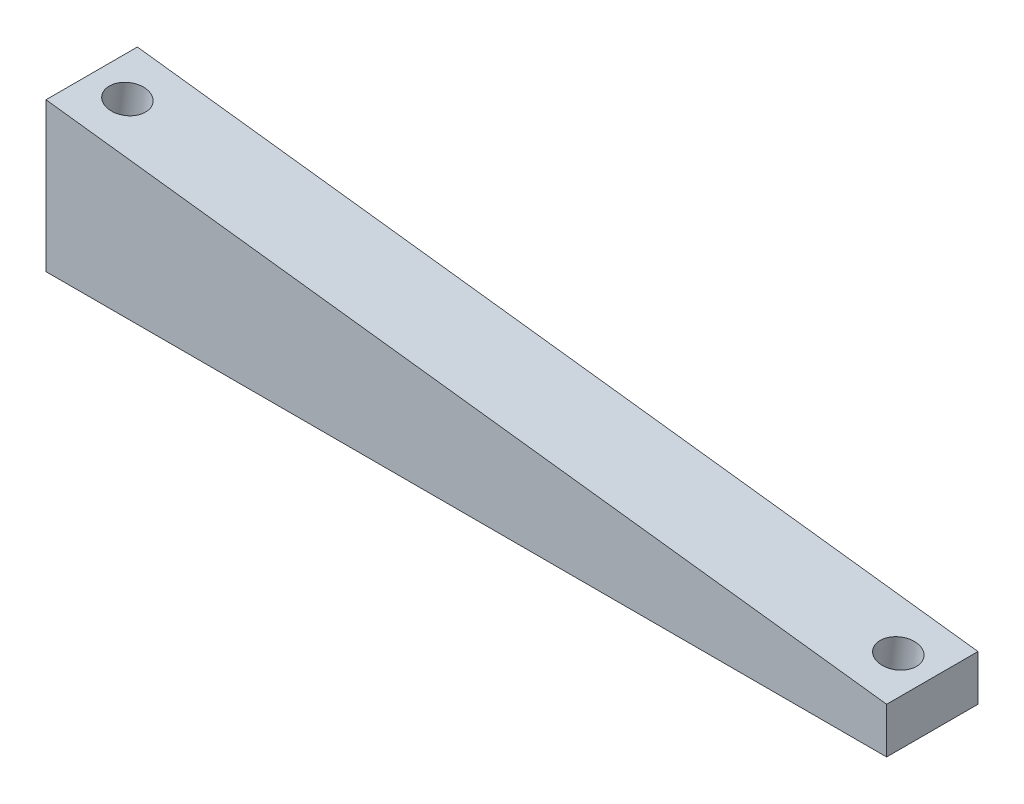
SolidWorks part; units mm, degrees
material "Plain Carbon Steel"
ref_plane "Front Plane" through (0, 0, 0) normal (0, 0, 1) x (1, 0, 0)
ref_plane "Top Plane" through (0, 0, 0) normal (0, 1, 0) x (1, 0, 0)
ref_plane "Right Plane" through (0, 0, 0) normal (1, 0, 0) x (0, 0, -1)
sketch "Sketch1" plane through (0, 0, 0) normal (0, 0, 1) x (1, 0, 0)
  line L0 (0, 0) -> (184, 0)
  line L1 (0, 0) -> (0, 32.5924)
  line L2 (184, 0) -> (184, 10)
  line L3 (184, 10) -> (0, 32.5924)
  dimension "D1" = 184
  dimension "D2" = 7
  dimension "D3" = 10
extrude "Boss-Extrude1" add sketch "Sketch1" along normal blind 20
sketch "Sketch2" plane through (3.9424, 32.1083, 0) normal (0.1219, 0.9925, 0) x (0.9925, -0.1219, 0)
  line L0 (181.4098, 0) -> (-3.972, 0) construction
  line L1 (181.4098, -20) -> (181.4098, 0) construction
  circle A0 centre (173.9098, -10) radius 4
  dimension "D2" = 8
  dimension "D1" = 10
  dimension "D3" = 7.5
extrude "Cut-Extrude1" cut sketch "Sketch2" against normal blind 15
pattern_linear "LPattern1" count 2 spacing 170 along (-0.9925, 0.1219, 0) of "Cut-Extrude1"
